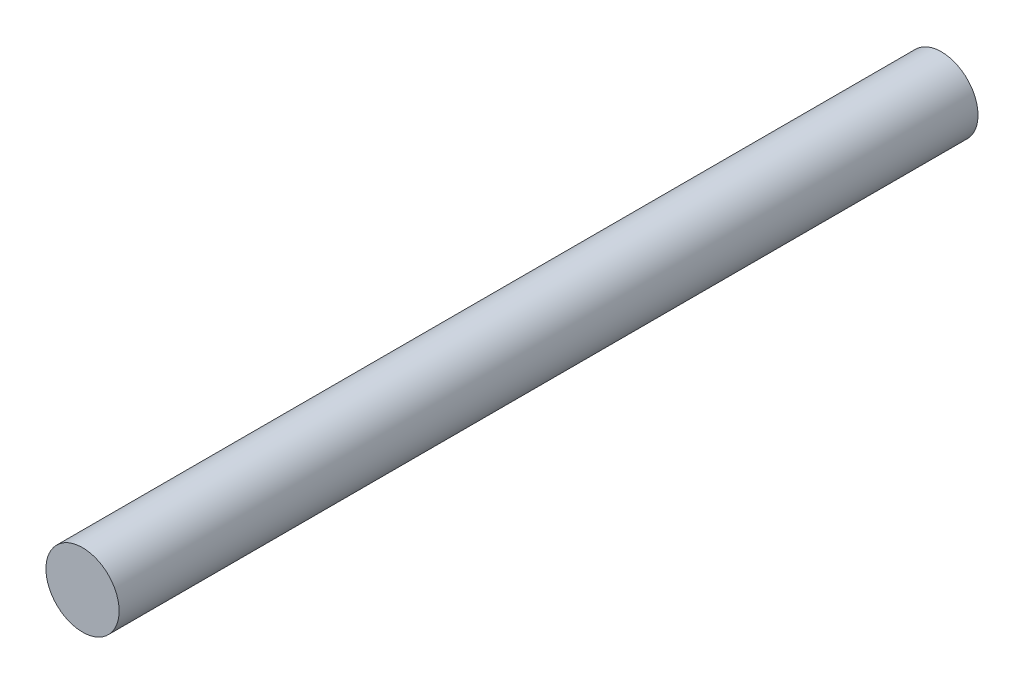
from build123d import *

# Parameters (mm, degrees)
SKETCH_1_R          = 15
EXTRUDE_1_DEPTH     = 400
CUT_EXTRUDE_START   = -48
SKETCH_2_R          = 15
CUT_EXTRUDE_1_DEPTH = 48


with BuildPart() as part:
    # 草图1 → 凸台-拉伸1 (new body)
    with BuildSketch(Plane.XY):
        Circle(SKETCH_1_R)
    extrude(amount=EXTRUDE_1_DEPTH)

    # 草图2 → 切除-拉伸1 (cut)
    with BuildSketch(Plane.XY.offset(400).offset(CUT_EXTRUDE_START)):
        Circle(SKETCH_2_R)
    extrude(amount=CUT_EXTRUDE_1_DEPTH, mode=Mode.SUBTRACT)


solid = part.part
